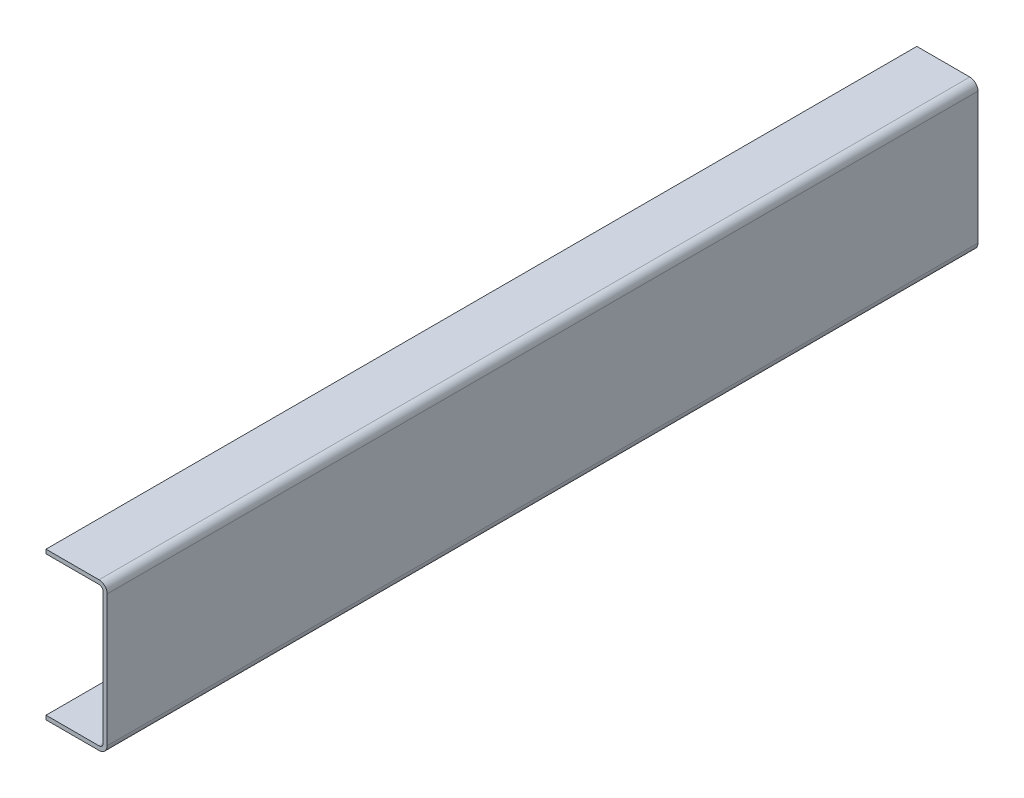
SolidWorks part; units mm, degrees
ref_plane "Front Plane" through (0, 0, 0) normal (0, 0, 1) x (1, 0, 0)
ref_plane "Top Plane" through (0, 0, 0) normal (0, 1, 0) x (1, 0, 0)
ref_plane "Right Plane" through (0, 0, 0) normal (1, 0, 0) x (0, 0, -1)
other "Configuration Table"
sketch "Sketch1" plane through (0, 0, 0) normal (0, 0, 1) x (1, 0, 0)
  line L0 (-60, -72.5) -> (-8, -72.5)
  line L1 (0, -64.5) -> (0, 64.5)
  line L2 (-8, 72.5) -> (-60, 72.5)
  line L3 (-60, 72.5) -> (-60, 68.5)
  line L4 (-60, 68.5) -> (-8, 68.5)
  line L5 (-4, 64.5) -> (-4, -64.5)
  line L6 (-8, -68.5) -> (-60, -68.5)
  line L7 (-60, -68.5) -> (-60, -72.5)
  arc A0 (-8, -72.5) -> (0, -64.5) centre (-8, -64.5) ccw
  arc A1 (0, 64.5) -> (-8, 72.5) centre (-8, 64.5) ccw
  arc A2 (-4, 64.5) -> (-8, 68.5) centre (-8, 64.5) ccw
  arc A3 (-8, -68.5) -> (-4, -64.5) centre (-8, -64.5) ccw
  dimension "D1" = 8
  dimension "D2" = 4
  dimension "D3" = 60
  dimension "D4" = 68.5
  dimension "D5" = 68.5
extrude "Boss-Extrude1" add sketch "Sketch1" along normal mid plane 854
